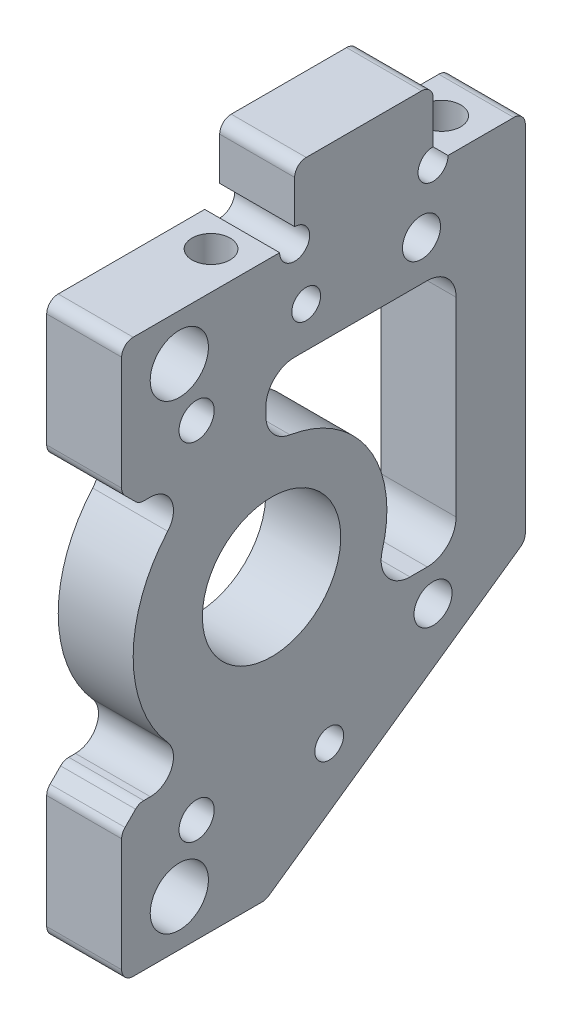
SolidWorks part; units mm, degrees
material "6061 合金"
ref_plane "前视基准面" through (0, 0, 0) normal (0, 0, 1) x (1, 0, 0)
ref_plane "上视基准面" through (0, 0, 0) normal (0, 1, 0) x (1, 0, 0)
ref_plane "右视基准面" through (0, 0, 0) normal (1, 0, 0) x (0, 0, -1)
sketch "草图1" plane through (0, 0, 0) normal (1, 0, 0) x (0, 0, -1)
  line L0 (-6, 0) -> (6, 0) construction
  line L1 (-13, 24) -> (-13, 11.25)
  line L2 (-13, 11.25) -> (-10.5089, 11.25)
  line L3 (-13, -11.25) -> (-10.5089, -11.25)
  line L4 (-13, -24) -> (-13, -11.25)
  line L5 (-13, -24) -> (-0.5, -24)
  line L6 (-13, 24) -> (0.7, 24)
  line L7 (2, 25.3) -> (2, 30)
  line L8 (2, 30) -> (14, 30)
  line L9 (14, 30) -> (14, 25.3)
  line L10 (15.3, 24) -> (22, 24)
  line L11 (-0.5, -24) -> (22, -8.2453)
  line L12 (22, -8.2453) -> (22, 24)
  line L13 (3, 19) -> (8, 19) construction
  line L14 (8, 19) -> (13, 19) construction
  line L16 (-0.5, 9.9875) -> (-0.5, 15.5)
  line L17 (-0.5, 15.5) -> (16, 15.5)
  line L18 (16, 15.5) -> (16, -6)
  line L19 (16, -6) -> (8, -6)
  line L20 (8, 30) -> (8, 19) construction
  circle A0 centre (0, 0) radius 6
  circle A1 centre (-6.5, 15) radius 1.525
  circle A2 centre (-8, 20) radius 2.525
  circle A3 centre (-6.5, -15) radius 1.525
  circle A4 centre (-8, -20) radius 2.525
  arc A5 (-9.0076, 7.9286) -> (-9.0076, -7.9286) centre (0, 0) ccw
  arc A6 (-10.5089, -11.25) -> (-9.0076, -7.9286) centre (-10.5089, -9.25) ccw
  arc A7 (-10.5089, 11.25) -> (-9.0076, 7.9286) centre (-10.5089, 9.25) cw
  arc A8 (0.7, 24) -> (2, 25.3) centre (2, 24) ccw
  arc A9 (14, 25.3) -> (15.3, 24) centre (14, 24) ccw
  circle A12 centre (3, 19) radius 1.5 construction
  circle A14 centre (5, -15) radius 1.5 construction
  arc A16 (-0.5, 9.9875) -> (8, -6) centre (0, 0) cw
  circle A17 centre (13, 19) radius 2 construction
  circle A18 centre (14, -9) radius 2 construction
  point P22 (-4.1758, -11.25)
  point P25 (-4.1758, 11.25)
  point P53 (14, 19)
  point P54 (0, 0)
  dimension "D1" = 12
  dimension "D2" = 15
  dimension "D4" = 3.05
  dimension "D5" = 5.05
  dimension "D8" = 13
  dimension "D9" = 2
  dimension "D10" = 12
  dimension "D14" = 1.3
  dimension "D15" = 3
  dimension "D19" = 9
  dimension "D22" = 5
  dimension "D24" = 10
  dimension "D30" = 4
  dimension "D3" = 6.5
  dimension "D6" = 8
  dimension "D7" = 20
  dimension "D11" = 22.5
  dimension "D12" = 24
  dimension "D13" = 6
  dimension "D16" = 22
  dimension "D17" = 6
  dimension "D18" = 3.5
  dimension "D20" = 8
  dimension "D21" = 12
  dimension "D23" = 5
  dimension "D25" = 6
  dimension "D26" = 18
  dimension "D27" = 5.5
  dimension "D28" = 145
  dimension "D29" = 9
  dimension "D31" = 5
  dimension "D32" = 9
  dimension "D33" = 6
extrude "凸台-拉伸1" add sketch "草图1" along normal blind 6.5
fillet "R2.5 圆角1" radius 2.5 5 edges at (3.25, -6, -8) (3.25, -6, -16) (3.25, 15.5, -16) (3.25, 15.5, 0.5) (3.25, 9.9875, 0.5)
sketch "草图2" plane through (6.5, 0, 0) normal (1, 0, 0) x (0, 0, -1)
  point P0 (5, -15)
  point P10 (3, 19)
hole_wizard "M3 螺纹孔1" positions "草图2" profile "草图3" tap size "M3" standard "GB" end condition through all
sketch "草图3" plane through (6.5, -15, -5) normal (0, 1, 0) x (0, 0, -1)
  line L0 (0, 0) -> (0, 6.5)
  line L1 (0, 6.5) -> (1.25, 6.5)
  line L2 (1.25, 6.5) -> (1.25, 0)
  line L5 (1.25, 0) -> (0, 0)
  line L11 (0, -6.35) -> (0, 107.95) construction
  dimension "通孔螺纹孔钻头直径" = 2.5
  dimension "通孔螺纹孔钻头深度" = 6.5
cosmetic thread "孔螺纹线1" parameters "D2"=3
cosmetic thread "孔螺纹线6" parameters "D2"=3
sketch "草图4" plane through (0, 24, 0) normal (0, 1, 0) x (1, 0, 0)
  line L0 (3.25, 22) -> (3.25, -13) construction
  line L1 (6.5, 22) -> (0, 22) construction
  line L2 (6.5, -13) -> (0, -13) construction
  line L3 (0, 8) -> (6.5, 8) construction
  line L4 (6.5, 14) -> (6.5, 2) construction
  line L6 (0, 14) -> (0, 2) construction
  point P6 (3.25, 18)
  point P16 (3.25, -2)
  point P26 (0, 8)
  dimension "D1" = 4
hole_wizard "M4 螺纹孔1" positions "草图4" profile "草图5" tap size "M4" standard "GB"
sketch "草图5" plane through (3.25, 24, 2) normal (1, 0, 0) x (0, 0, 1)
  line L0 (0, 0) -> (0, 7.9914)
  line L1 (0, 7.9914) -> (1.65, 7)
  line L2 (1.65, 7) -> (1.65, 0)
  line L5 (1.65, 0) -> (0, 0)
  line L10 (0, 7.9914) -> (-1.65, 7) construction
  line L11 (0, -6.35) -> (0, 107.95) construction
  dimension "螺纹孔钻头直径" = 3.3
  dimension "螺纹孔钻头深度" = 7
  dimension "导头角度" = 118
cosmetic thread "孔螺纹线7" parameters "D1"=8, "D2"=4
cosmetic thread "孔螺纹线8" parameters "D1"=8, "D2"=4
sketch "草图6" plane through (6.5, 0, 0) normal (1, 0, 0) x (0, 0, -1)
  point P0 (14, -9)
  point P2 (13, 19)
hole_wizard "M4 螺纹孔2" positions "草图6" profile "草图7" tap size "M4" standard "GB" end condition through all
sketch "草图7" plane through (6.5, -9, -14) normal (0, 1, 0) x (0, 0, -1)
  line L0 (0, 0) -> (0, 6.5)
  line L1 (0, 6.5) -> (1.65, 6.5)
  line L2 (1.65, 6.5) -> (1.65, 0)
  line L5 (1.65, 0) -> (0, 0)
  line L11 (0, -6.35) -> (0, 107.95) construction
  dimension "通孔螺纹孔钻头直径" = 3.3
  dimension "通孔螺纹孔钻头深度" = 6.5
cosmetic thread "孔螺纹线9" parameters "D2"=4
cosmetic thread "孔螺纹线10" parameters "D2"=4
chamfer "C1.5 倒角1" distance 1.5 angle 45 2 edges at (3.25, -11.25, 13) (3.25, 11.25, 13)
fillet "R1 圆角2" radius 1 11 edges at (3.25, -24, 0.5) (3.25, -8.2453, -22) (3.25, 24, 13) (3.25, 24, -22) (3.25, 30, -14) (3.25, 30, -2) (3.25, -24, 13) (3.25, -12.75, 13) (3.25, -11.25, 11.5) (3.25, 12.75, 13) (3.25, 11.25, 11.5)
